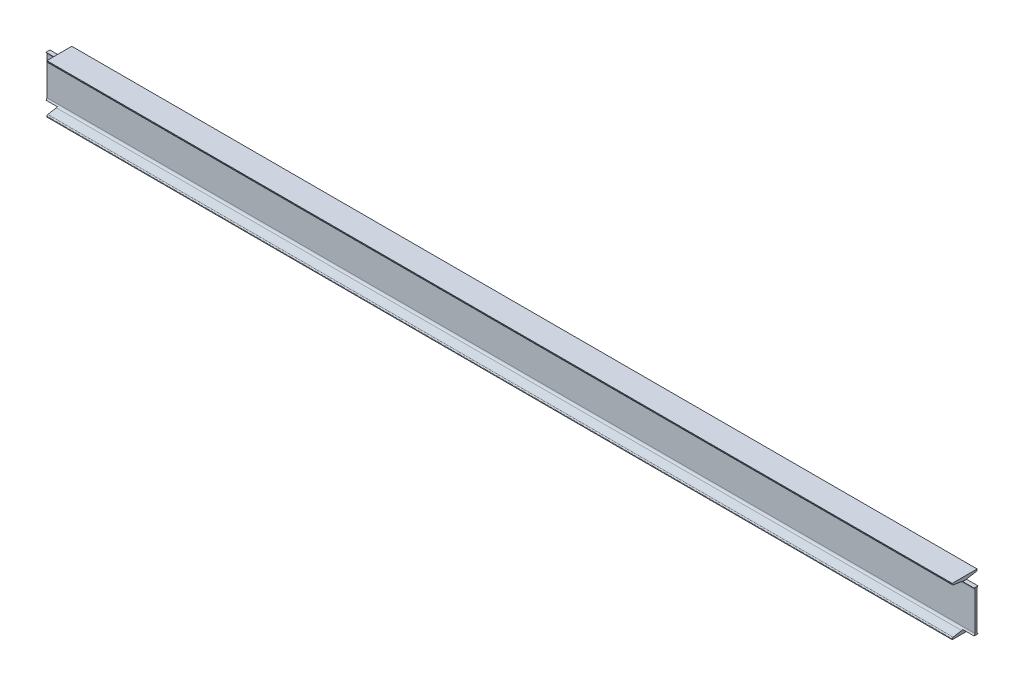
SolidWorks part; units mm, degrees
ref_plane "Front" through (0, 0, 0) normal (0, 0, 1) x (1, 0, 0)
ref_plane "Top" through (0, 0, 0) normal (0, 1, 0) x (1, 0, 0)
ref_plane "Right" through (0, 0, 0) normal (1, 0, 0) x (0, 0, -1)
sketch "Sketch1" plane through (0, 0, 0) normal (1, 0, 0) x (0, 0, -1)
  line L0 (-51, 0) -> (51, 0)
  line L1 (0, 106.3348) -> (0, -35.2641) construction
  line L2 (-4.5, 185.475) -> (-4.5, 14.525)
  line L3 (-4.5, 14.525) -> (-51, 6.775)
  line L4 (-51, 6.775) -> (-51, 0)
  line L5 (-51, 6.775) -> (-4.5, 6.775) construction
  line L6 (-4.5, 6.775) -> (-4.5, 14.525) construction
  line L7 (-23.25, 200) -> (-23.25, 0) construction
  line L8 (-51, 200) -> (51, 200)
  line L9 (-51, 200) -> (-51, 193.225)
  line L10 (-51, 193.225) -> (-4.5, 185.475)
  line L11 (-51, 193.225) -> (-4.5, 193.225) construction
  line L12 (-4.5, 193.225) -> (-4.5, 185.475) construction
  line L13 (-23.25, 11.4) -> (-23.25, 0) construction
  line L14 (-23.25, 200) -> (-23.25, 188.6) construction
  line L15 (51, 6.775) -> (51, 0)
  line L16 (4.5, 14.525) -> (51, 6.775)
  line L17 (4.5, 185.475) -> (4.5, 14.525)
  line L18 (51, 193.225) -> (4.5, 185.475)
  line L19 (51, 200) -> (51, 193.225)
  point P22 (0, 200)
extrude "Base" add sketch "Sketch1" along normal blind 3800
fillet "Fillet1" radius 9 4 edges at (1900, 185.475, -4.5) (1900, 14.525, -4.5) (1900, 14.525, 4.5) (1900, 185.475, 4.5)
fillet "Fillet2" radius 4.5 4 edges at (1900, 193.225, 51) (1900, 6.775, 51) (1900, 6.775, -51) (1900, 193.225, -51)
sketch "草图1" plane through (0, 200, 0) normal (0, 1, 0) x (1, 0, 0)
  line L0 (3800, 51) -> (0, 51) construction
  line L1 (0, -51) -> (46.5, -51)
  line L2 (0, -51) -> (0, 51)
  line L3 (0, 51) -> (46.5, 51)
  line L4 (46.5, -51) -> (46.5, 51)
  line L5 (3800, -51) -> (0, -51) construction
  line L6 (3800, 51) -> (3753.5, 51)
  line L7 (3800, 51) -> (3800, -51)
  line L8 (3800, -51) -> (3753.5, -51)
  line L9 (3753.5, 51) -> (3753.5, -51)
  dimension "D1" = 46.5
  dimension "D2" = 46.5
extrude "Cut-Extrude1" cut sketch "草图1" against normal blind 15
sketch "Sketch2" plane through (0, 0, 0) normal (0, -1, 0) x (-1, 0, 0)
  line L0 (-3800, 51) -> (0, 51) construction
  line L1 (0, -51) -> (-46.5, -51)
  line L2 (0, -51) -> (0, 51)
  line L3 (0, 51) -> (-46.5, 51)
  line L4 (-46.5, -51) -> (-46.5, 51)
  line L6 (-3800, -51) -> (-3753.5, -51)
  line L7 (-3800, -51) -> (-3800, 51)
  line L8 (-3800, 51) -> (-3753.5, 51)
  line L9 (-3753.5, -51) -> (-3753.5, 51)
  dimension "D1" = 46.5
  dimension "D2" = 46.5
extrude "Cut-Extrude2" cut sketch "Sketch2" against normal blind 15
equation "\"D5@Sketch1\" =  ( \"b@Sketch1\" - \"d@Sketch1\" ) /12"
equation "\"D10@Sketch1\" = \"D5@Sketch1\""
equation "\"t1@Sketch1\" = \"t@Sketch1\""
equation "\"D6@Sketch1\" =  ( \"b@Sketch1\" - \"d@Sketch1\" ) /4"
